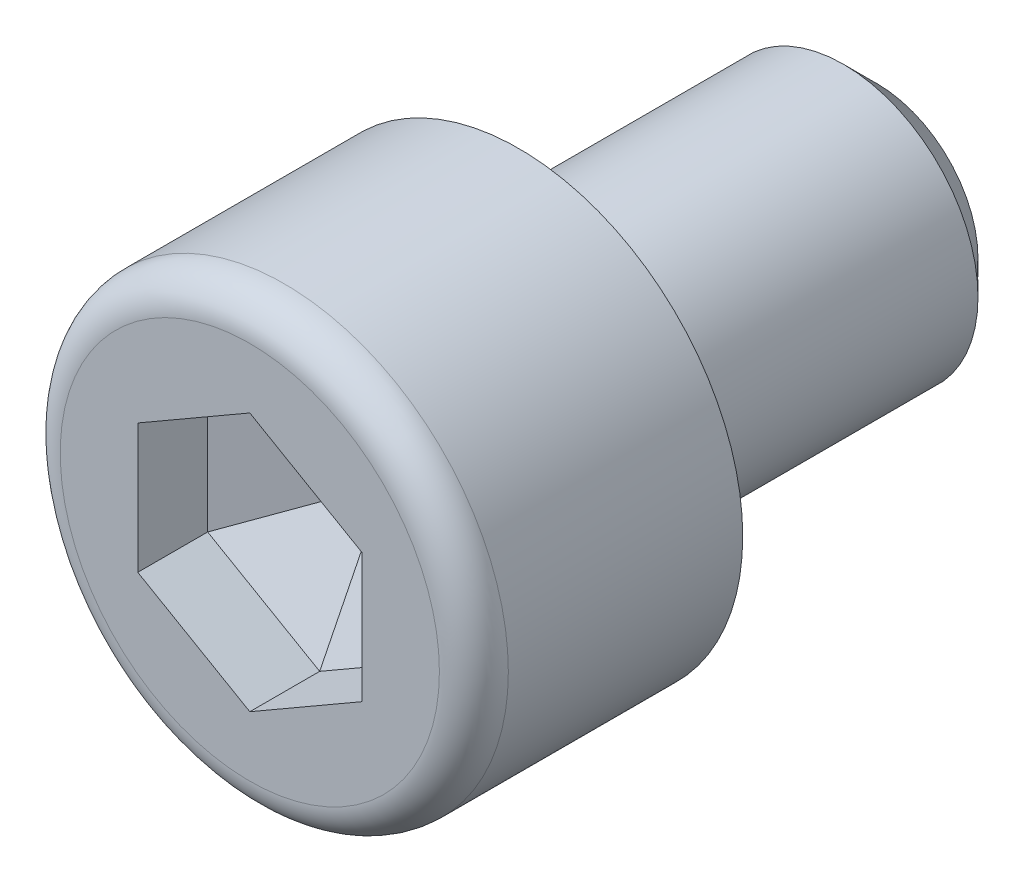
from build123d import *
from OCP.BRepFilletAPI import BRepFilletAPI_MakeChamfer

# Parameters (mm, degrees)
SKETCH_1_R          = 5
EXTRUDE_1_DEPTH     = 6
CUT_EXTRUDE_1_DEPTH = 3
SKETCH_3_R          = 3
EXTRUDE_2_DEPTH     = 8
CHAMFER_1_SIZE      = 0.75
FILLET_1_R          = 0.769230769
CHAMFER_2_SIZE      = 1.44092219
CHAMFER_2_SIZE2     = 2.495750443
FILLET_2_R          = 0.1


with BuildPart() as part:
    # 草图1 → 凸台-拉伸1 (new body)
    with BuildSketch(Plane.XY):
        Circle(SKETCH_1_R)
    extrude(amount=EXTRUDE_1_DEPTH)

    # 草图2 → 切除-拉伸1 (cut)
    with BuildSketch(Plane.XY.offset(6)):
        Polygon((2.5, 1.443375673), (0, 2.886751346), (-2.5, 1.443375673), (-2.5, -1.443375673), (0, -2.886751346), (2.5, -1.443375673), align=None)
    extrude(amount=-CUT_EXTRUDE_1_DEPTH, mode=Mode.SUBTRACT)

    # 草图3 → 凸台-拉伸2 (add)
    with BuildSketch(Plane(origin=(0, 0, 0), x_dir=(-1, 0, 0), z_dir=(0, 0, -1))):
        with Locations(Location((0, 0, 0), (0, 0, 180))):
            Circle(SKETCH_3_R)
    extrude(amount=EXTRUDE_2_DEPTH)

    # 倒角1
    chamfer_1_edges = [part.edges().sort_by_distance(p)[0] for p in [
        (-3, 0, -8),
    ]]
    chamfer(chamfer_1_edges, length=CHAMFER_1_SIZE)

    # 圆角1
    fillet_1_edges = [part.edges().sort_by_distance(p)[0] for p in [
        (-5, 0, 6),
    ]]
    fillet(fillet_1_edges, radius=FILLET_1_R)

    # 倒角2: one chamfer whose edges measure the first distance from different faces: ONE call of the kernel's chamfer builder (chamfer() names one face for all edges)
    chamfer_2_edges_1 = [part.edges().sort_by_distance(p)[0] for p in [
        (1.25, 2.165063509, 3),
    ]]
    chamfer_2_side_1 = [part.faces().sort_by_distance(p)[0] for p in [
        (1.25, 2.165063509, 4.5),
    ]]
    chamfer_2_edges_2 = [part.edges().sort_by_distance(p)[0] for p in [
        (2.5, 0, 3),
    ]]
    chamfer_2_side_2 = [part.faces().sort_by_distance(p)[0] for p in [
        (2.5, 0, 4.5),
    ]]
    chamfer_2_edges_3 = [part.edges().sort_by_distance(p)[0] for p in [
        (1.25, -2.165063509, 3),
    ]]
    chamfer_2_side_3 = [part.faces().sort_by_distance(p)[0] for p in [
        (1.25, -2.165063509, 4.5),
    ]]
    chamfer_2_edges_4 = [part.edges().sort_by_distance(p)[0] for p in [
        (-1.25, -2.165063509, 3),
    ]]
    chamfer_2_side_4 = [part.faces().sort_by_distance(p)[0] for p in [
        (-1.25, -2.165063509, 4.5),
    ]]
    chamfer_2_edges_5 = [part.edges().sort_by_distance(p)[0] for p in [
        (-2.5, 0, 3),
    ]]
    chamfer_2_side_5 = [part.faces().sort_by_distance(p)[0] for p in [
        (-2.5, 0, 4.5),
    ]]
    chamfer_2_edges_6 = [part.edges().sort_by_distance(p)[0] for p in [
        (-1.25, 2.165063509, 3),
    ]]
    chamfer_2_side_6 = [part.faces().sort_by_distance(p)[0] for p in [
        (-1.25, 2.165063509, 4.5),
    ]]
    chamfer_2 = BRepFilletAPI_MakeChamfer(part.part.solid().wrapped)
    for e in chamfer_2_edges_1:
        chamfer_2.Add(CHAMFER_2_SIZE, CHAMFER_2_SIZE2, e.wrapped, chamfer_2_side_1[0].wrapped)  # the first distance lies on this face
    for e in chamfer_2_edges_2:
        chamfer_2.Add(CHAMFER_2_SIZE, CHAMFER_2_SIZE2, e.wrapped, chamfer_2_side_2[0].wrapped)  # the first distance lies on this face
    for e in chamfer_2_edges_3:
        chamfer_2.Add(CHAMFER_2_SIZE, CHAMFER_2_SIZE2, e.wrapped, chamfer_2_side_3[0].wrapped)  # the first distance lies on this face
    for e in chamfer_2_edges_4:
        chamfer_2.Add(CHAMFER_2_SIZE, CHAMFER_2_SIZE2, e.wrapped, chamfer_2_side_4[0].wrapped)  # the first distance lies on this face
    for e in chamfer_2_edges_5:
        chamfer_2.Add(CHAMFER_2_SIZE, CHAMFER_2_SIZE2, e.wrapped, chamfer_2_side_5[0].wrapped)  # the first distance lies on this face
    for e in chamfer_2_edges_6:
        chamfer_2.Add(CHAMFER_2_SIZE, CHAMFER_2_SIZE2, e.wrapped, chamfer_2_side_6[0].wrapped)  # the first distance lies on this face
    add(Compound.cast(chamfer_2.Shape()), mode=Mode.REPLACE)

    # 圆角2
    fillet_2_edges = [part.edges().sort_by_distance(p)[0] for p in [
        (-3, 0, 0),
    ]]
    fillet(fillet_2_edges, radius=FILLET_2_R)


solid = part.part
